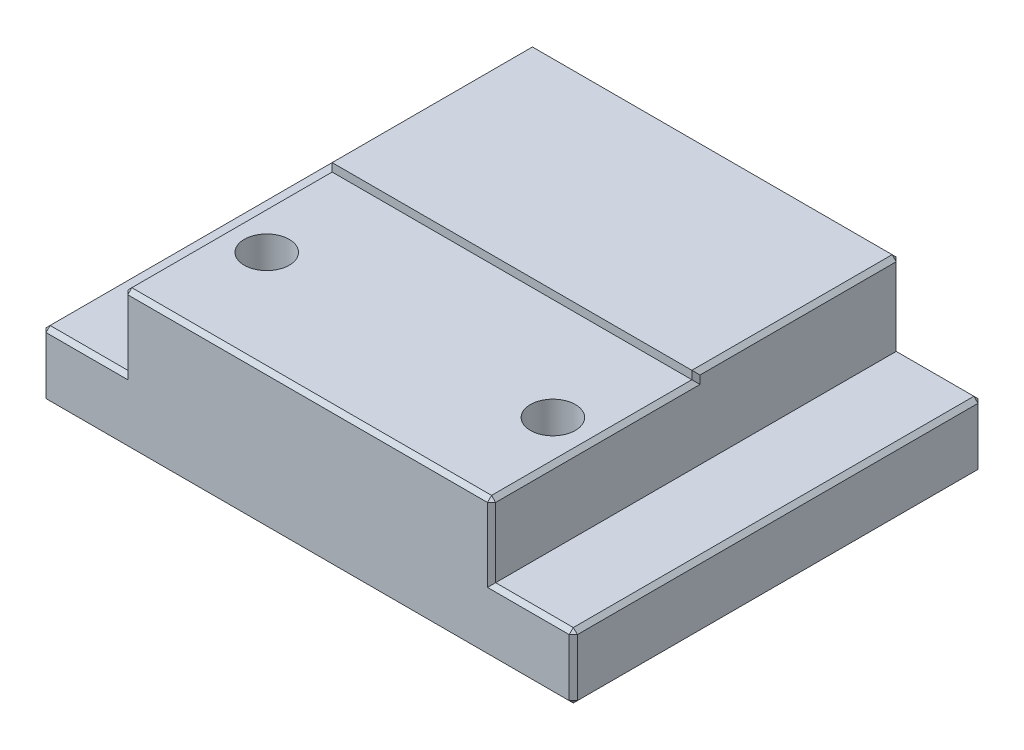
SolidWorks part; units mm, degrees
ref_plane "Front Plane" through (0, 0, 0) normal (0, 0, 1) x (1, 0, 0)
ref_plane "Top Plane" through (0, 0, 0) normal (0, 1, 0) x (1, 0, 0)
ref_plane "Right Plane" through (0, 0, 0) normal (1, 0, 0) x (0, 0, -1)
other "Configuration Table"
sketch "Sketch2" plane through (0, 0, 0) normal (0, 0, 1) x (1, 0, 0)
  line L0 (55, 8) -> (65, 8)
  line L1 (0, 0) -> (65, 0)
  line L2 (0, 0) -> (0, 8)
  line L3 (0, 8) -> (10, 8)
  line L4 (65, 0) -> (65, 8)
  line L5 (10, 18) -> (55, 18)
  line L6 (10, 18) -> (10, 8)
  line L8 (55, 18) -> (55, 8)
  dimension "D1" = 65
  dimension "D2" = 8
  dimension "D3" = 45
  dimension "D4" = 10
  dimension "D5" = 18
extrude "Boss-Extrude1" add sketch "Sketch2" along normal blind 50
sketch "Sketch3" plane through (0, 0, 0) normal (0, -1, 0) x (1, 0, 0)
  line L0 (55, 50) -> (10, 50) construction
  line L1 (55, 0) -> (10, 0) construction
  line L3 (32.5, 50) -> (32.5, 0) construction
  point P7 (50, 37.5)
  point P8 (15, 37.5)
  dimension "D1" = 12.5
  dimension "D2" = 35
  dimension "D3" = 17.5
hole_wizard "CBORE for M5 Slotted cheese head screws1" positions "Sketch3" profile "Sketch4" counterbore size "M5" standard "GB" end condition through all
sketch "Sketch4" plane through (15, 0, 37.5) normal (1, 0, 0) x (0, 0, -1)
  line L0 (0, 0) -> (0, 18)
  line L1 (0, 18) -> (2.75, 18)
  line L3 (2.75, 18) -> (2.75, 6)
  line L4 (5, 6) -> (2.75, 6)
  line L5 (5, 6) -> (5, 0.025)
  line L6 (5, 0.025) -> (5.025, 0)
  line L7 (5.025, 0) -> (0, 0)
  line L8 (-5, 0.025) -> (-5.025, 0) construction
  line L11 (0, -6.35) -> (0, 107.95) construction
  dimension "通孔孔直径" = 5.5
  dimension "通孔孔深度" = 18
  dimension "柱形沉头孔直径" = 10
  dimension "柱形沉头孔深度" = 6
  dimension "近端锥形沉头孔直径" = 10.05
  dimension "近端锥形沉头孔角度" = 90
sketch "Sketch6" plane through (0, 18, 0) normal (0, 1, 0) x (1, 0, 0)
  line L0 (55, -50) -> (55, 0) construction
  line L1 (10, -50) -> (55, -50)
  line L2 (10, -50) -> (10, -25)
  line L3 (10, -25) -> (55, -25)
  line L4 (55, -50) -> (55, -25)
  dimension "D1" = 25
extrude "Cut-Extrude1" cut sketch "Sketch6" against normal blind 1
chamfer "Chamfer1" distance 0.5 29 edges at (10, 8, 25) (10, 17.5, 25) (10, 17, 37.5) (55, 8, 25) (55, 17, 37.5) (55, 17.5, 25) (55, 18, 12.5) (32.5, 18, 25) (10, 18, 12.5) (65, 0, 25) (65, 8, 25) (0, 8, 25) (32.5, 0, 0) (65, 4, 0) (60, 8, 0) (55, 13, 0) (32.5, 18, 0) (10, 13, 0) (5, 8, 0) (0, 4, 0) (0, 0, 25) (60, 8, 50) (65, 4, 50) (32.5, 0, 50) (0, 4, 50) (5, 8, 50) (10, 12.5, 50) (32.5, 17, 50) (55, 12.5, 50)
